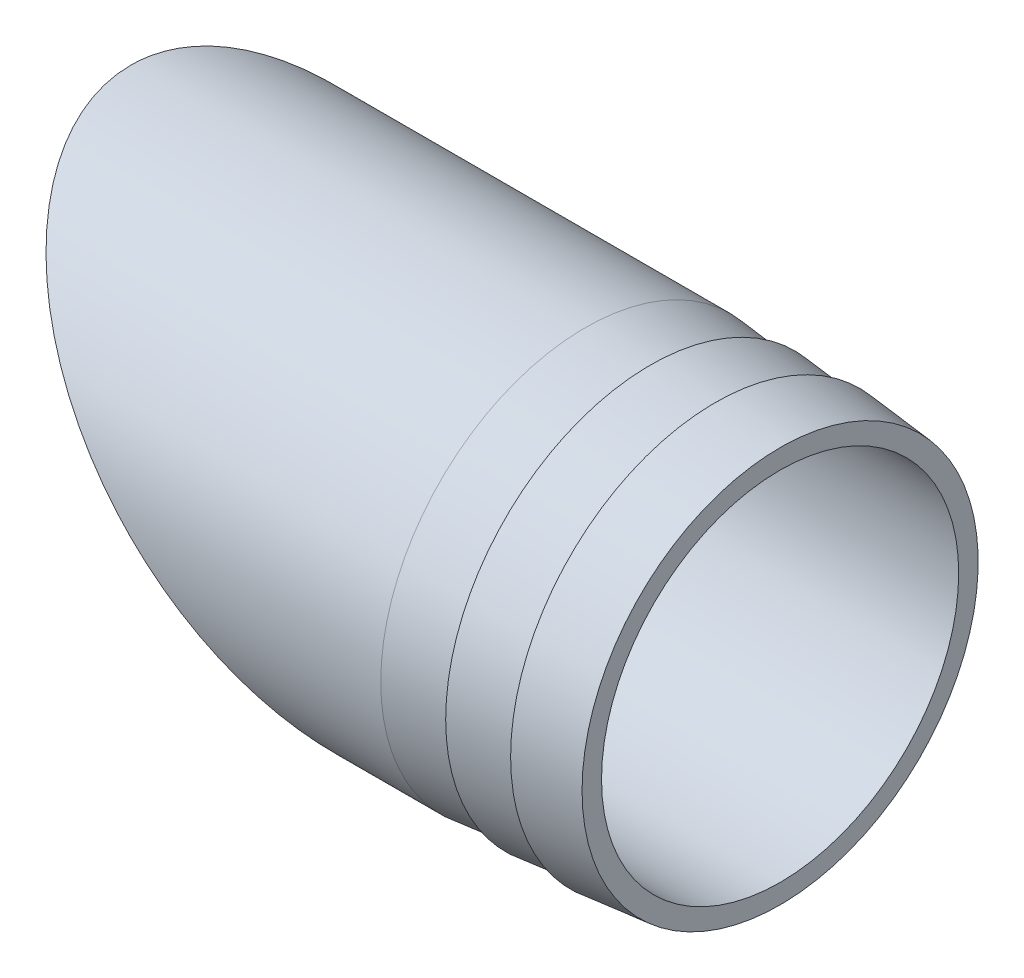
from build123d import *

# Parameters (mm, degrees)
CUT_EXTRUDE1_DEPTH      = 110.473741144
CUT_EXTRUDE1_DEPTH_BACK = 110.473741144


with BuildPart() as part:
    # Sketch1 → Revolve1 (revolve)
    with BuildSketch(Plane.XY, mode=Mode.PRIVATE) as revolve1_sk:
        Polygon((0, 27.5), (0, 31.5), (70, 31.5), (80, 30.5), (80, 31.5), (90, 30.5), (90, 31.5), (100, 30.5), (100, 27.5), align=None)
    revolve(revolve1_sk.sketch.rotate(Axis((0, 0, 0), (1, 0, 0)), 90), axis=Axis((0, 0, 0), (1, 0, 0)))

    # Sketch2 → Cut-Extrude1 (cut, two sides: drawn at the far end of the back side and taken through both)
    with BuildSketch(Plane.XY.offset(-CUT_EXTRUDE1_DEPTH_BACK)):
        Polygon((-199.7384521, 231.2384521), (0, 31.5), (96.333692144, -64.833692144), (296.072144244, -264.572144244), (-103.404759956, -664.049048445), (-599.2153563, -168.2384521), align=None)
    extrude(amount=CUT_EXTRUDE1_DEPTH + CUT_EXTRUDE1_DEPTH_BACK, mode=Mode.SUBTRACT)


solid = part.part
